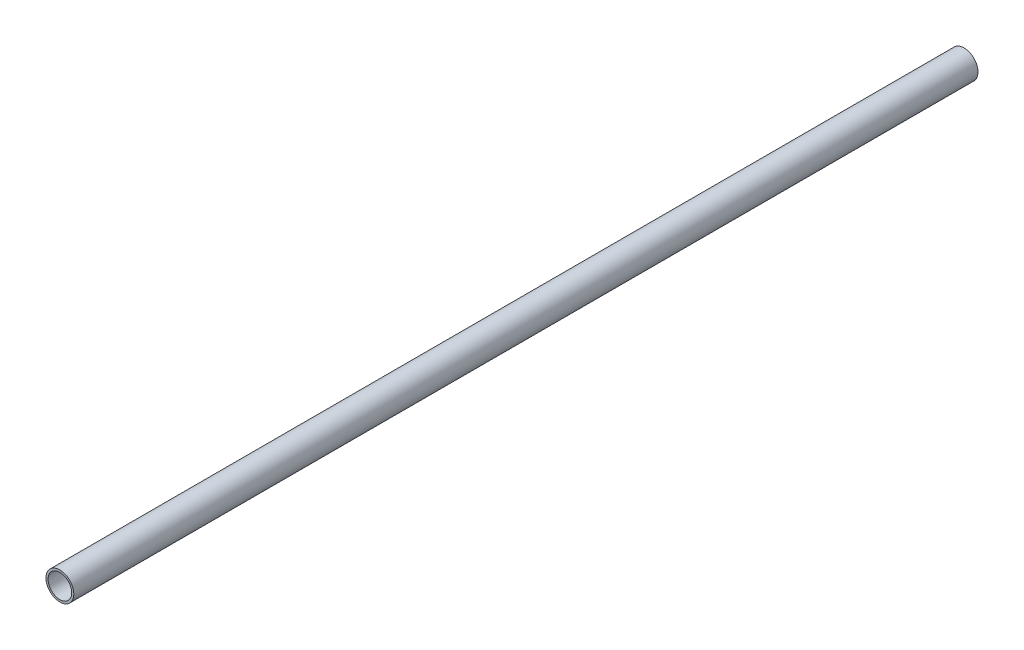
from build123d import *

# Parameters (mm, degrees)
SKETCH1_R           = 20
SKETCH1_R_2         = 17
BOSS_EXTRUDE1_DEPTH = 650


with BuildPart() as part:
    # Sketch1 → Boss-Extrude1 (new, symmetric)
    with BuildSketch(Plane.XY):
        Circle(SKETCH1_R)
        Circle(SKETCH1_R_2, mode=Mode.SUBTRACT)
    extrude(amount=BOSS_EXTRUDE1_DEPTH, both=True)


solid = part.part
